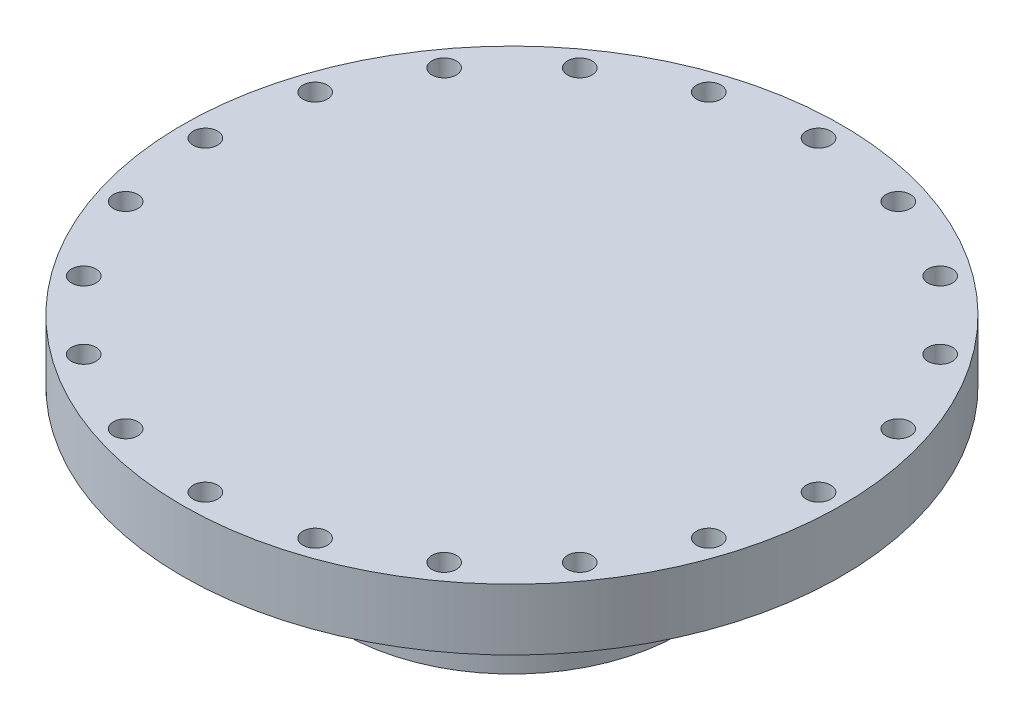
from build123d import *

# Parameters (mm, degrees)
SKETCH1_R                  = 215
BOSS_EXTRUDE1_DEPTH        = 40
F_16_0_16_DIAMETER_HOLE1_D = 16
SKETCH7_R                  = 110
SKETCH7_R_2                = 40
BOSS_EXTRUDE2_DEPTH        = 85


with BuildPart() as part:
    # Sketch1 → Boss-Extrude1 (new body)
    with BuildSketch(Plane(origin=(0, 0, 0), x_dir=(1, 0, 0), z_dir=(0, 1, 0))):
        with Locations(Location((0, 0, 0), (0, 0, 270))):
            Circle(SKETCH1_R)
    extrude(amount=BOSS_EXTRUDE1_DEPTH)

    # Ø16.0 (16) Diameter Hole1 (through all)
    with Locations(Plane(origin=(0, 40, 0), x_dir=(1, 0, 0), z_dir=(0, 1, 0))):
        with Locations((200, 0), (190.211303259, -61.803398875), (161.803398875, -117.557050458), (117.557050458, -161.803398875), (61.803398875, -190.211303259), (0, -200), (-61.803398875, -190.211303259), (-117.557050458, -161.803398875), (-161.803398875, -117.557050458), (-190.211303259, -61.803398875), (-200, 0), (-190.211303259, 61.803398875), (-161.803398875, 117.557050458), (-117.557050458, 161.803398875), (-61.803398875, 190.211303259), (0, 200), (61.803398875, 190.211303259), (117.557050458, 161.803398875), (161.803398875, 117.557050458), (190.211303259, 61.803398875)):
            Hole(F_16_0_16_DIAMETER_HOLE1_D / 2)

    # Sketch7 → Boss-Extrude2 (add)
    with BuildSketch(Plane.XZ):
        with Locations(Location((0, 0, 0), (0, 0, 90))):
            Circle(SKETCH7_R)
        with Locations(Location((0, 0, 0), (0, 0, 270))):
            Circle(SKETCH7_R_2, mode=Mode.SUBTRACT)
    extrude(amount=BOSS_EXTRUDE2_DEPTH)


solid = part.part
